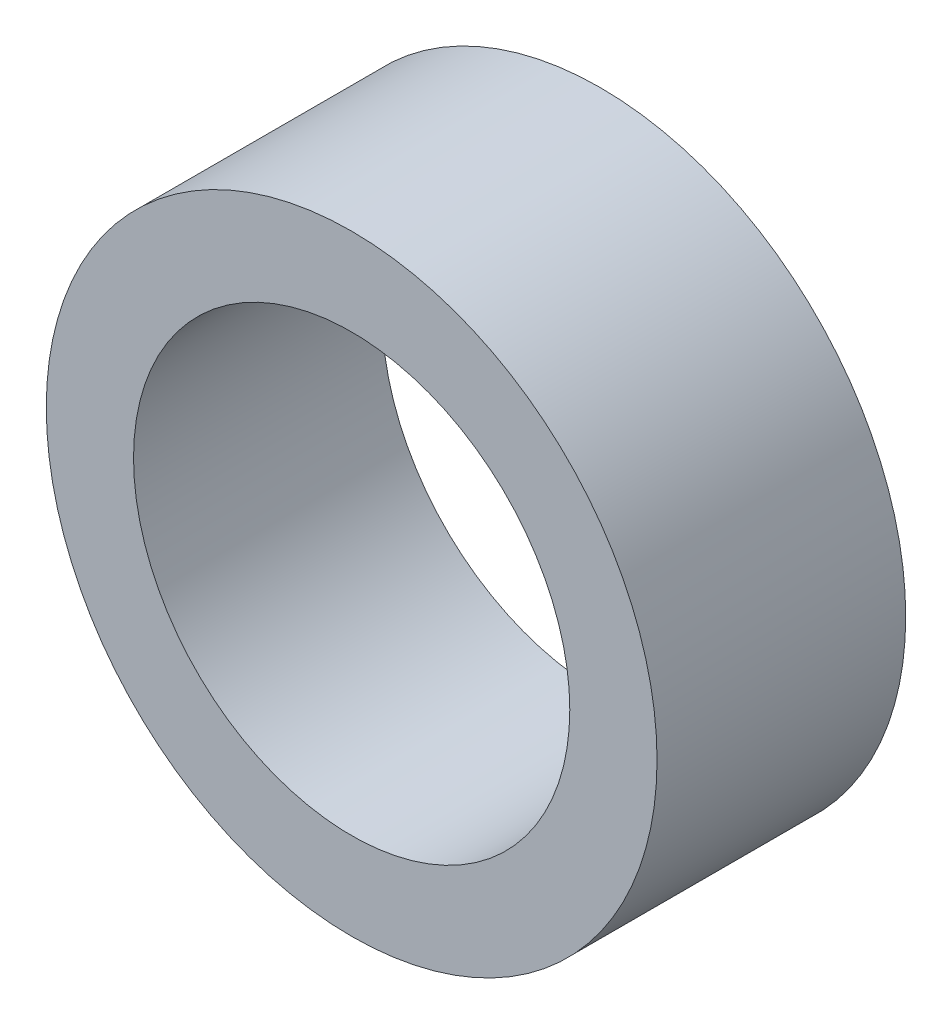
SolidWorks part; units mm, degrees
ref_plane "前视基准面" through (0, 0, 0) normal (0, 0, 1) x (1, 0, 0)
ref_plane "上视基准面" through (0, 0, 0) normal (0, 1, 0) x (1, 0, 0)
ref_plane "右视基准面" through (0, 0, 0) normal (1, 0, 0) x (0, 0, -1)
sketch "草图1" plane through (0, 0, 0) normal (0, 0, 1) x (1, 0, 0)
  circle A0 centre (0, 0) radius 5
  circle A1 centre (0, 0) radius 7
  dimension "D1" = 10
  dimension "D2" = 14
extrude "凸台-拉伸1" add sketch "草图1" along normal blind 5.7
